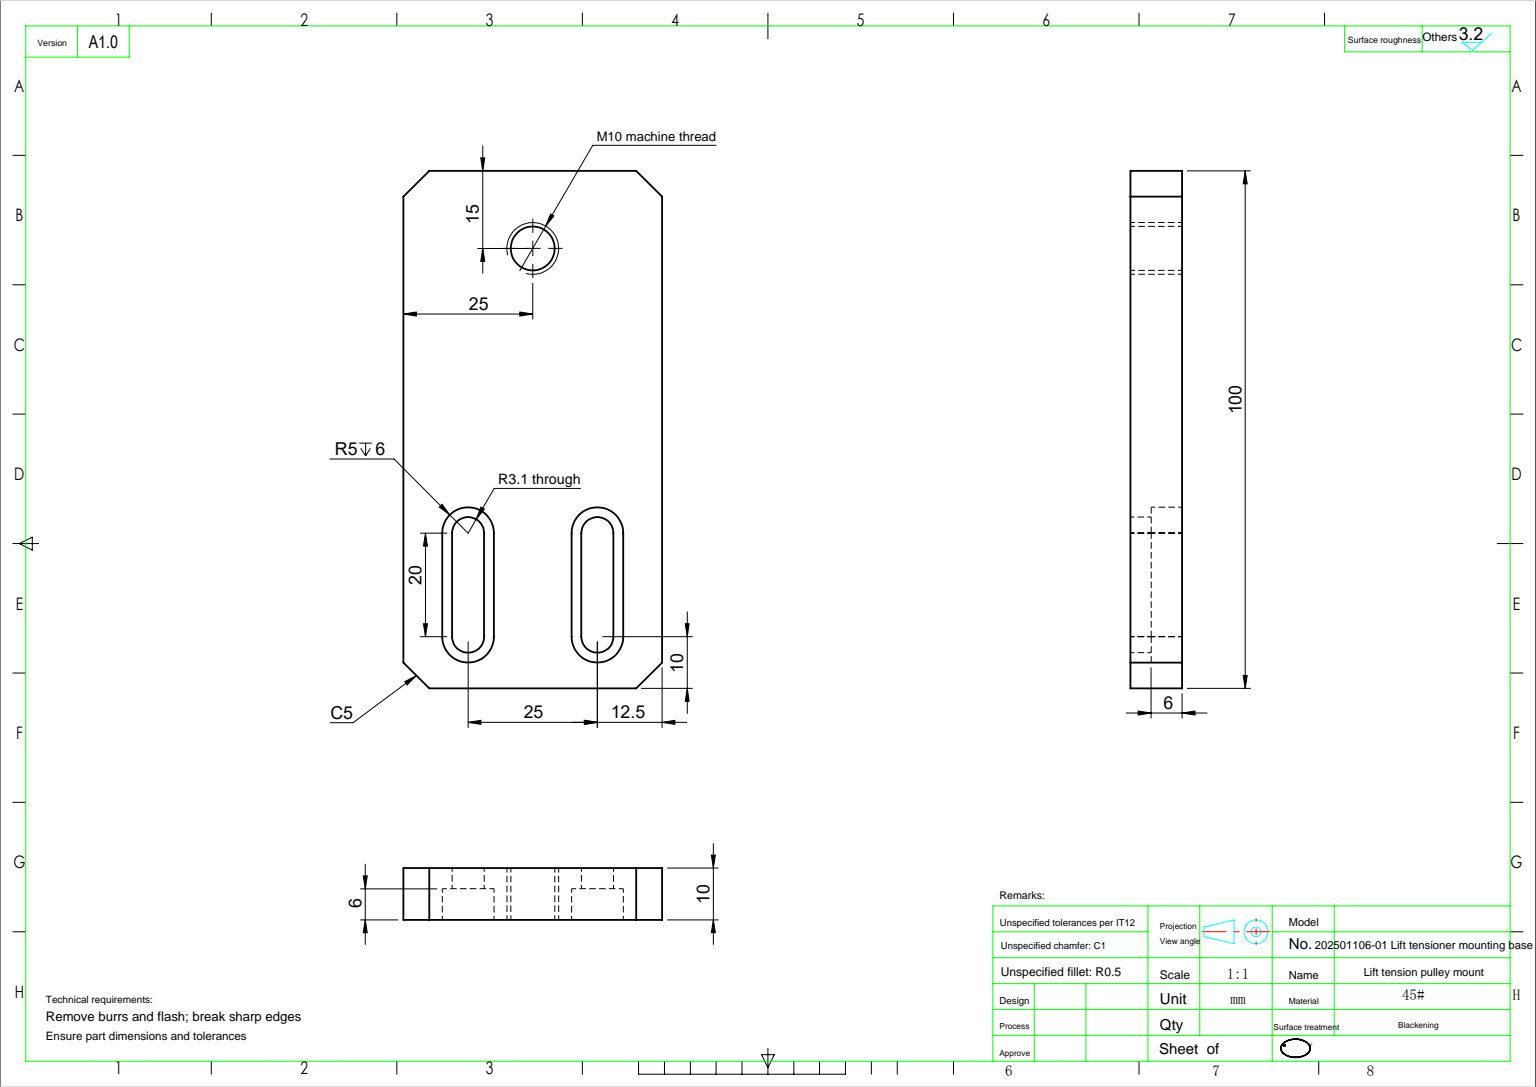
from build123d import *

# Parameters (mm, degrees)
SKETCH_1_W          = 50
SKETCH_1_H          = 100
EXTRUDE_1_DEPTH     = 10
CUT_EXTRUDE_1_DEPTH = 10
CUT_EXTRUDE_2_DEPTH = 6
CHAMFER_1_SIZE      = 5
SKETCH_4_R          = 4.25
CUT_EXTRUDE_3_DEPTH = 10


with BuildPart() as part:
    # 草图1 → 凸台-拉伸1 (new body)
    with BuildSketch(Plane.XY):
        Rectangle(SKETCH_1_W, SKETCH_1_H)
    extrude(amount=EXTRUDE_1_DEPTH)

    # 草图2 → 切除-拉伸1 (cut)
    with BuildSketch(Plane.XY.offset(10)):
        with BuildLine():
            Line((-9.4, -20), (-9.4, -40))
            ThreePointArc((-9.4, -40), (-12.5, -43.1), (-15.6, -40))
            Line((-15.6, -40), (-15.6, -20))
            ThreePointArc((-15.6, -20), (-12.5, -16.9), (-9.4, -20))
        make_face()
        with BuildLine():
            Line((9.4, -40), (9.4, -20))
            ThreePointArc((9.4, -20), (12.5, -16.9), (15.6, -20))
            Line((15.6, -20), (15.6, -40))
            ThreePointArc((15.6, -40), (12.5, -43.1), (9.4, -40))
        make_face()
    extrude(amount=-CUT_EXTRUDE_1_DEPTH, mode=Mode.SUBTRACT)

    # 草图3 → 切除-拉伸2 (cut)
    with BuildSketch(Plane.XY.offset(10)):
        with BuildLine():
            Line((-7.5, -20), (-7.5, -40))
            ThreePointArc((-7.5, -40), (-12.5, -45), (-17.5, -40))
            Line((-17.5, -40), (-17.5, -20))
            ThreePointArc((-17.5, -20), (-12.5, -15), (-7.5, -20))
        make_face()
        with BuildLine():
            Line((17.5, -20), (17.5, -40))
            ThreePointArc((17.5, -40), (12.5, -45), (7.5, -40))
            Line((7.5, -40), (7.5, -20))
            ThreePointArc((7.5, -20), (12.5, -15), (17.5, -20))
        make_face()
    extrude(amount=-CUT_EXTRUDE_2_DEPTH, mode=Mode.SUBTRACT)

    # 倒角1
    chamfer_1_edges = [part.edges().sort_by_distance(p)[0] for p in [
        (25, -50, 5),
        (-25, -50, 5),
        (-25, 50, 5),
        (25, 50, 5),
    ]]
    chamfer(chamfer_1_edges, length=CHAMFER_1_SIZE)

    # 草图4 → 切除-拉伸3 (cut)
    with BuildSketch(Plane.XY.offset(10)):
        with Locations((0, 35)):
            Circle(SKETCH_4_R)
    extrude(amount=-CUT_EXTRUDE_3_DEPTH, mode=Mode.SUBTRACT)


solid = part.part
